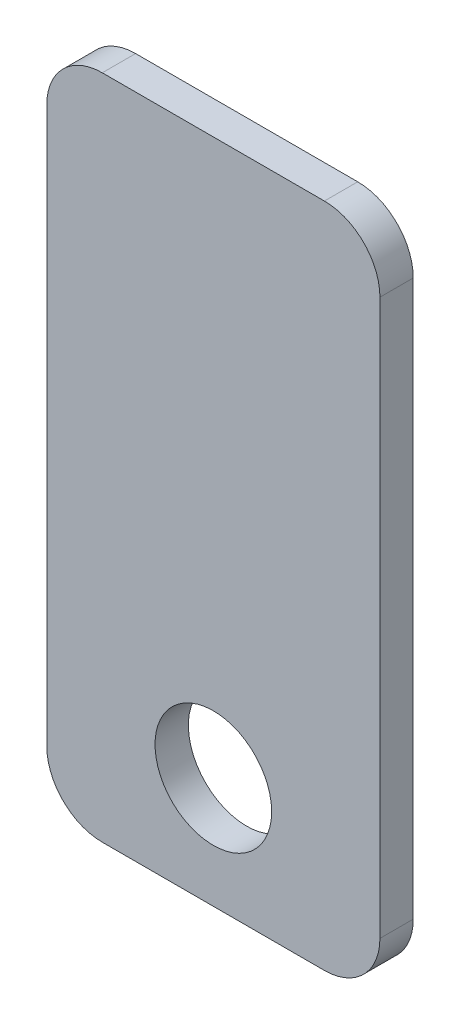
SolidWorks part; units mm, degrees
material "1023 碳钢板 (SS)"
ref_plane "Front Plane" through (0, 0, 0) normal (0, 0, 1) x (1, 0, 0)
ref_plane "Top Plane" through (0, 0, 0) normal (0, 1, 0) x (1, 0, 0)
ref_plane "Right Plane" through (0, 0, 0) normal (1, 0, 0) x (0, 0, -1)
sketch "Sketch1" plane through (0, 0, 0) normal (0, 0, 1) x (1, 0, 0)
  line L1 (-10, 30) -> (10, 30)
  line L2 (-15, 25) -> (-15, -25)
  line L3 (-10, -30) -> (10, -30)
  line L4 (15, 25) -> (15, -25)
  line L5 (-15, 30) -> (15, -30) construction
  line L6 (-15, -30) -> (15, 30) construction
  arc A0 (10, 30) -> (15, 25) centre (10, 25) cw
  arc A1 (-15, -25) -> (-10, -30) centre (-10, -25) ccw
  arc A2 (-10, 30) -> (-15, 25) centre (-10, 25) ccw
  arc A3 (10, -30) -> (15, -25) centre (10, -25) ccw
  circle A4 centre (0, -20) radius 5.25
  point P0 (0, 0)
  dimension "D3" = 5
  dimension "D4" = 10
  dimension "D1" = 30
  dimension "D2" = 60
extrude "Boss-Extrude1" add sketch "Sketch1" along normal blind 3
